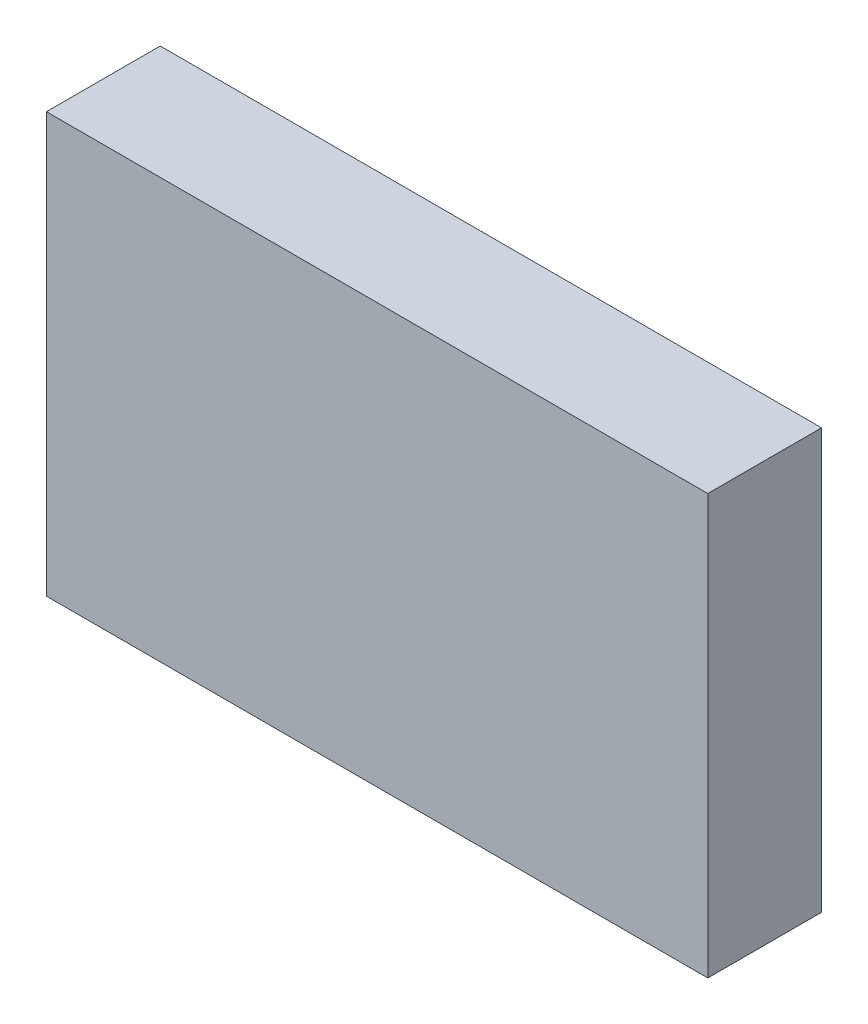
SolidWorks part; units mm, degrees
material "普通碳钢"
ref_plane "前视基准面" through (0, 0, 0) normal (0, 0, 1) x (1, 0, 0)
ref_plane "上视基准面" through (0, 0, 0) normal (0, 1, 0) x (1, 0, 0)
ref_plane "右视基准面" through (0, 0, 0) normal (1, 0, 0) x (0, 0, -1)
sketch "草图1" plane through (0, 0, 0) normal (0, 0, 1) x (1, 0, 0)
  line L1 (-232.5, -147.5) -> (232.5, -147.5)
  line L2 (-232.5, -147.5) -> (-232.5, 147.5)
  line L3 (-232.5, 147.5) -> (232.5, 147.5)
  line L4 (232.5, -147.5) -> (232.5, 147.5)
  line L5 (-232.5, -147.5) -> (232.5, 147.5) construction
  line L6 (-232.5, 147.5) -> (232.5, -147.5) construction
  point P0 (0, 0)
  dimension "D1" = 465
  dimension "D2" = 295
extrude "凸台-拉伸1" add sketch "草图1" along normal blind 80
